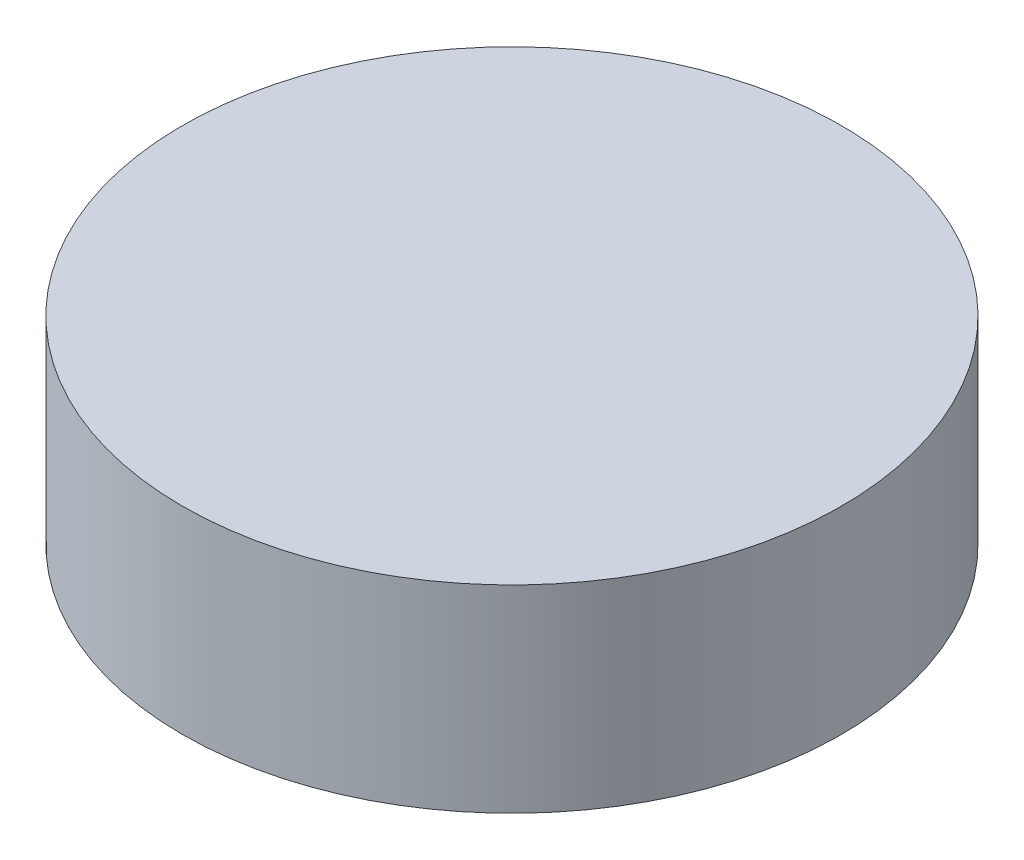
from build123d import *

# Parameters (mm, degrees)
SKETCH1_R           = 10
BOSS_EXTRUDE1_DEPTH = 6


with BuildPart() as part:
    # Sketch1 → Boss-Extrude1 (new body)
    with BuildSketch(Plane(origin=(0, 0, 0), x_dir=(1, 0, 0), z_dir=(0, 1, 0))):
        with Locations(Location((0, 0, 0), (0, 0, 270))):
            Circle(SKETCH1_R)
    extrude(amount=BOSS_EXTRUDE1_DEPTH)


solid = part.part
